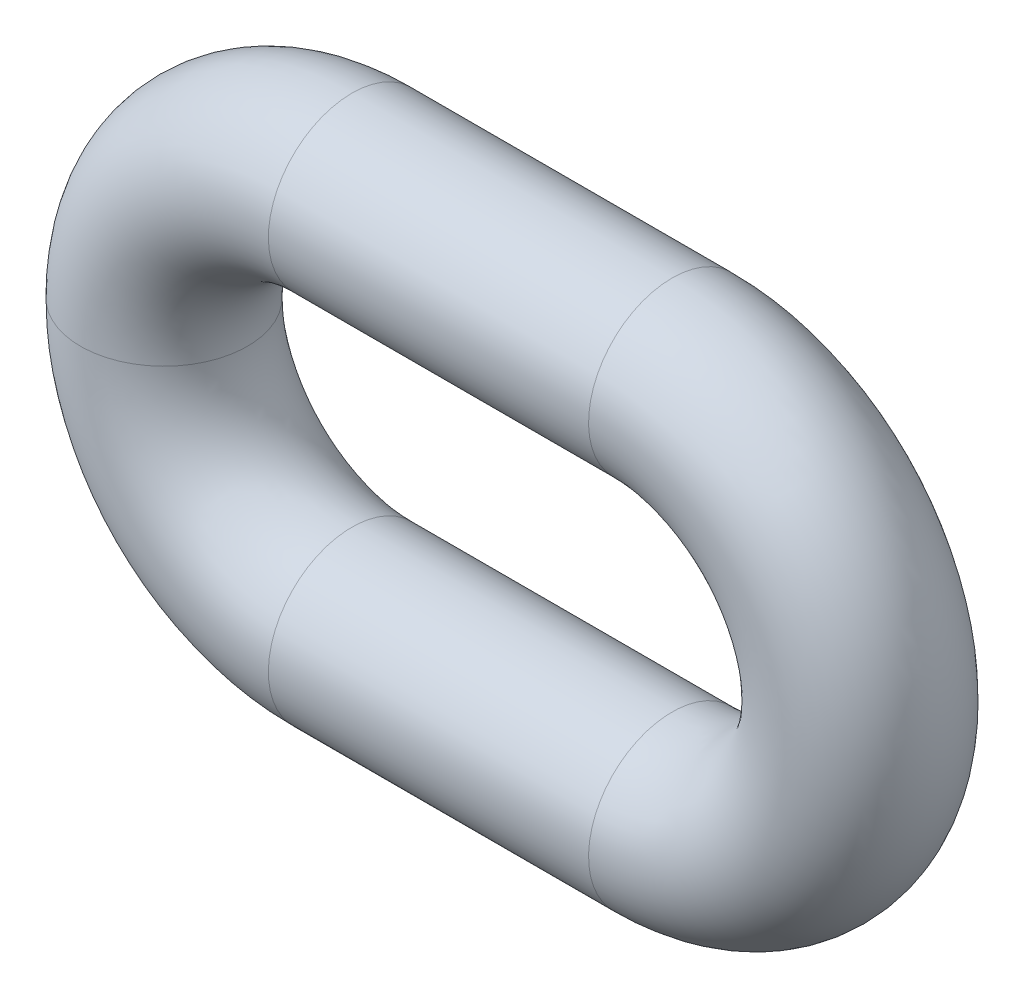
SolidWorks part; units mm, degrees
material "1.7147 (20MnCr5)"
ref_plane "前视基准面" through (0, 0, 0) normal (0, 0, 1) x (1, 0, 0)
ref_plane "上视基准面" through (0, 0, 0) normal (0, 1, 0) x (1, 0, 0)
ref_plane "右视基准面" through (0, 0, 0) normal (1, 0, 0) x (0, 0, -1)
sketch "草图1" plane through (0, 0, 0) normal (0, 0, 1) x (1, 0, 0)
  line L0 (0, 78) -> (92, 78)
  line L1 (0, -78) -> (92, -78)
  line L2 (-78, 0) -> (170, 0) construction
  line L3 (0, 0) -> (92, 0) construction
  line L7 (92, 0) -> (0, 0) construction
  line L10 (-78, 0) -> (-76, 0) construction
  line L11 (76, 0) -> (170, 0) construction
  arc A0 (0, 78) -> (0, -78) centre (0, 0) ccw
  arc A1 (92, -78) -> (92, 78) centre (92, 0) ccw
  point P11 (0, 0)
  dimension "D1" = 248
  dimension "D2" = 78
sketch "草图18" plane through (0, 0, 0) normal (0, 1, 0) x (1, 0, 0)
  line L0 (-78, 0) -> (170, 0) construction
  line L3 (-54, 0) -> (-78, 0) construction
  line L4 (-54, 0) -> (-30, 0) construction
  line L5 (-78, 0) -> (0, 0) construction
  circle A0 centre (-54, 0) radius 24
  dimension "D1" = 48
sweep "扫描2" add profiles "草图18" path "草图1"
sketch "草图23" plane through (0, 0, 0) normal (0, 1, 0) x (1, 0, 0)
  line L0 (-54, 0) -> (146, 0) construction
  line L1 (-30, 0) -> (0, 0) construction
  line L2 (-6, 0) -> (-30, 0) construction
  circle A0 centre (-54, 0) radius 48
  circle A1 centre (-54, 0) radius 24 construction
  circle A2 centre (146, 0) radius 54
  circle A3 centre (-54, 0) radius 24 construction
  dimension "D1" = 24
  dimension "D2" = 108
sketch "草图24" plane through (0, 0, 0) normal (0, 0, 1) x (1, 0, 0)
  line L0 (-54, 0) -> (146, 0) construction
  line L1 (-30, 0) -> (-6, 0) construction
  line L2 (46, 30) -> (46, 0) construction
  line L3 (0, 30) -> (92, 30) construction
  circle A2 centre (-6, 0) radius 24
  circle A3 centre (98, 0) radius 24
  dimension "D1" = 48
  dimension "D2" = 24
  dimension "D3" = 76
